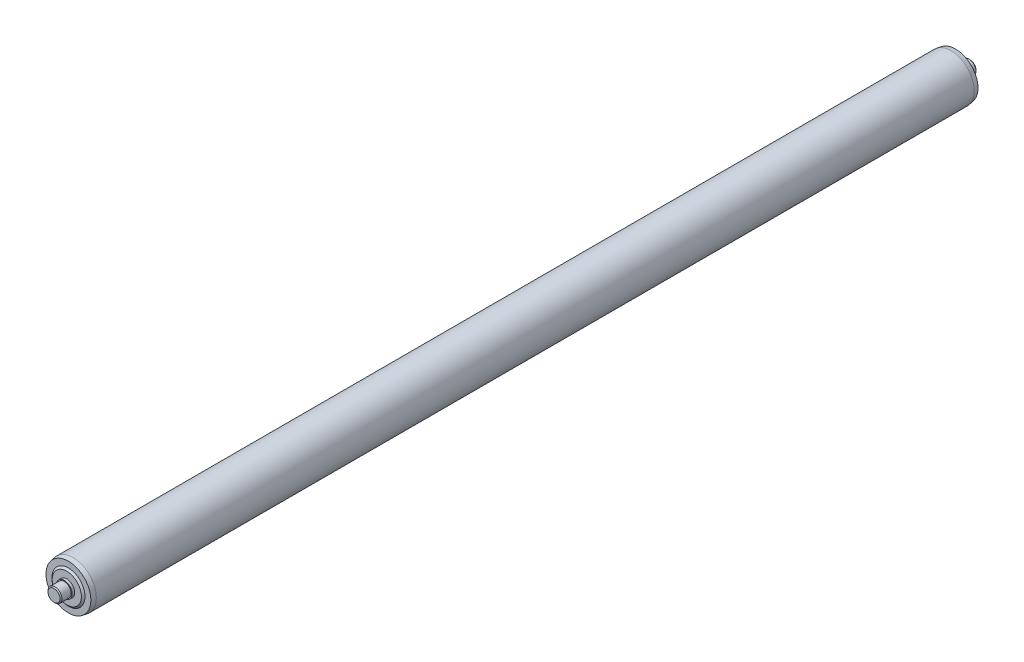
from build123d import *

# Parameters (mm, degrees)
CHAMFER1_SIZE  = 5
CHAMFER1_SIZE2 = 0.881634904
CHAMFER2_SIZE  = 1


with BuildPart() as part:
    # Sketch3 → Revolve1 (revolve)
    with BuildSketch(Plane(origin=(0, 0, 0), x_dir=(0, 0, -1), z_dir=(1, 0, 0)), mode=Mode.PRIVATE) as revolve1_sk:
        Polygon((-325, 25), (629, 25), (629, 17.799192231), (630.760753628, 15.700807769), (630.760753628, 8.5), (633.5, 8.5), (633.5, 7.5), (644.5, 7.5), (644.5, 0), (-340.5, 0), (-340.5, 7.5), (-329.5, 7.5), (-329.5, 8.5), (-326.760753628, 8.5), (-326.760753628, 15.700807769), (-325, 17.799192231), align=None)
    revolve(revolve1_sk.sketch.rotate(Axis((0, 0, 340.5), (0, 0, -1)), 90), axis=Axis((0, 0, 340.5), (0, 0, -1)))

    # Chamfer1
    chamfer1_edges = [part.edges().sort_by_distance(p)[0] for p in [
        (-25, 0, -629),
        (-25, 0, 325),
    ]]
    chamfer1_side = [part.faces().sort_by_distance(p)[0] for p in [
        (-25, 0, -152),
    ]]
    chamfer(chamfer1_edges, length=CHAMFER1_SIZE, length2=CHAMFER1_SIZE2, reference=chamfer1_side[0])

    # Chamfer2
    chamfer2_edges = [part.edges().sort_by_distance(p)[0] for p in [
        (-7.5, 0, 340.5),
        (-7.5, 0, -644.5),
    ]]
    chamfer(chamfer2_edges, length=CHAMFER2_SIZE)


solid = part.part
